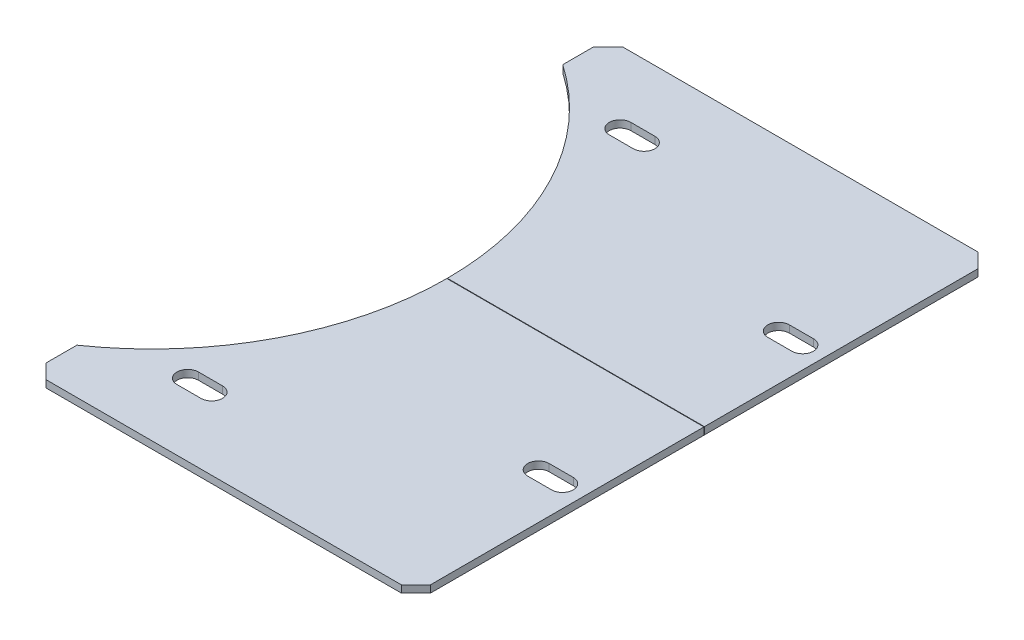
SolidWorks part; units mm, degrees
ref_plane "Front Plane" through (0, 0, 0) normal (0, 0, 1) x (1, 0, 0)
ref_plane "Top Plane" through (0, 0, 0) normal (0, 1, 0) x (1, 0, 0)
ref_plane "Right Plane" through (0, 0, 0) normal (1, 0, 0) x (0, 0, -1)
sketch "Sketch1" plane through (0, 0, 0) normal (0, 1, 0) x (1, 0, 0)
  line L1 (-276, 60) -> (276, 60)
  line L2 (-276, 60) -> (-276, -60)
  line L3 (-276, -60) -> (276, -60)
  line L4 (276, 60) -> (276, -60)
  line L5 (-276, 60) -> (276, -60) construction
  line L6 (-276, -60) -> (276, 60) construction
  point P0 (0, 0)
  dimension "D1" = 120
  dimension "D2" = 552
extrude "Boss-Extrude1" add sketch "Sketch1" along normal blind 1.5
chamfer "Chamfer1" distance 3 angle 45 2 edges at (276, 0.75, -60) (276, 0.75, 60)
chamfer "Chamfer2" distance 3 angle 45 2 edges at (-276, 0.75, -60) (-276, 0.75, 60)
sketch "Sketch12" plane through (0, 1.5, 0) normal (0, 1, 0) x (1, 0, 0)
  line L0 (-258.5, 45) -> (-253.5, 45) construction
  line L1 (-258.5, 47.25) -> (-253.5, 47.25)
  line L2 (-258.5, 42.75) -> (-253.5, 42.75)
  line L3 (-258.5, -45) -> (-253.5, -45) construction
  line L4 (-258.5, -42.75) -> (-253.5, -42.75)
  line L5 (-258.5, -47.25) -> (-253.5, -47.25)
  line L6 (0, 0) -> (-462.1641, 0) construction
  line L7 (-276, 57) -> (-276, -57) construction
  line L8 (273, 60) -> (-273, 60) construction
  arc A0 (-258.5, 47.25) -> (-258.5, 42.75) centre (-258.5, 45) ccw
  arc A1 (-253.5, 42.75) -> (-253.5, 47.25) centre (-253.5, 45) ccw
  arc A2 (-258.5, -42.75) -> (-258.5, -47.25) centre (-258.5, -45) ccw
  arc A3 (-253.5, -47.25) -> (-253.5, -42.75) centre (-253.5, -45) ccw
  point P2 (-256, 45)
  point P7 (-256, -45)
  dimension "D1" = 4.5
  dimension "D2" = 5
  dimension "D3" = 20
  dimension "D4" = 15
extrude "Cut-Extrude6" cut sketch "Sketch12" against normal through all
sketch "Sketch13" plane through (0, 1.5, 0) normal (0, 1, 0) x (1, 0, 0)
  line L0 (276, -57) -> (276, 57) construction
  line L1 (-276, 0.05) -> (276, 0.05)
  line L2 (-276, 0.05) -> (-276, -0.05)
  line L3 (-276, -0.05) -> (276, -0.05)
  line L4 (276, 0.05) -> (276, -0.05)
  line L5 (-276, 0.05) -> (276, -0.05) construction
  line L6 (-276, -0.05) -> (276, 0.05) construction
  line L7 (-276, 57) -> (-276, -57) construction
  point P0 (0, 0)
  dimension "D1" = 0.1
extrude "Cut-Extrude7" cut sketch "Sketch13" against normal through all
sketch "Sketch15" plane through (0, 1.5, 0) normal (0, 1, 0) x (1, 0, 0)
  line L0 (-276, -0.05) -> (276, -0.05) construction
  line L1 (52, 35.95) -> (-14, 35.95)
  line L2 (55, 32.95) -> (55, -33.05)
  line L3 (52, -36.05) -> (-14, -36.05)
  line L4 (-17, 32.95) -> (-17, -33.05)
  line L5 (55, 35.95) -> (-17, -36.05) construction
  line L6 (55, -36.05) -> (-17, 35.95) construction
  line L7 (-276, 57) -> (-276, 0.05) construction
  arc A0 (-17, -33.05) -> (-14, -36.05) centre (-14, -33.05) ccw
  arc A1 (55, -33.05) -> (52, -36.05) centre (52, -33.05) cw
  arc A2 (55, 32.95) -> (52, 35.95) centre (52, 32.95) ccw
  arc A3 (-14, 35.95) -> (-17, 32.95) centre (-14, 32.95) ccw
  point P0 (19, -0.05)
  dimension "D3" = 3
  dimension "D1" = 72
  dimension "D2" = 72
  dimension "D4" = 295
extrude "Cut-Extrude9" cut sketch "Sketch15" against normal through all
sketch "Sketch16" plane through (0, 1.5, 0) normal (0, 1, 0) x (1, 0, 0)
  line L0 (276, 0.05) -> (276, 57) construction
  line L1 (0, 0) -> (352.5911, 0) construction
  line L2 (0, 0) -> (0, 143.0362) construction
  circle A0 centre (311, 0) radius 61.5
  circle A1 centre (-311, 0) radius 61.5
  dimension "D1" = 123
  dimension "D2" = 35
extrude "Cut-Extrude10" cut sketch "Sketch16" against normal blind 10
sketch "Sketch17" plane through (0, 0, 0) normal (0, -1, 0) x (1, 0, 0)
  line L0 (-200.5, -25) -> (-205.5, -25) construction
  line L1 (-200.5, -27.25) -> (-205.5, -27.25)
  line L2 (-200.5, -22.75) -> (-205.5, -22.75)
  line L3 (-200.5, 25) -> (-205.5, 25) construction
  line L4 (-200.5, 22.75) -> (-205.5, 22.75)
  line L5 (-200.5, 27.25) -> (-205.5, 27.25)
  line L6 (-203, -60) -> (-203, 60) construction
  line L8 (273, -60) -> (-273, -60) construction
  line L9 (-273, 60) -> (273, 60) construction
  line L10 (-311, 0) -> (-268.0046, 0) construction
  line L11 (-276, -57) -> (-276, -50.5693) construction
  arc A0 (-200.5, -27.25) -> (-200.5, -22.75) centre (-200.5, -25) ccw
  arc A1 (-205.5, -22.75) -> (-205.5, -27.25) centre (-205.5, -25) ccw
  arc A2 (-200.5, 22.75) -> (-200.5, 27.25) centre (-200.5, 25) ccw
  arc A3 (-205.5, 27.25) -> (-205.5, 22.75) centre (-205.5, 25) ccw
  point P2 (-203, -25)
  point P7 (-203, 25)
  dimension "D1" = 5
  dimension "D2" = 4.5
  dimension "D3" = 50
  dimension "D4" = 73
sketch "Sketch18" plane through (0, 0, 0) normal (0, -1, 0) x (1, 0, 0)
  line L0 (-276, -57) -> (-276, -50.5693) construction
  line L1 (802.7899, 126.4319) -> (-196, 126.4319)
  line L2 (802.7899, 126.4319) -> (802.7899, -126.4319)
  line L3 (802.7899, -126.4319) -> (-196, -126.4319)
  line L4 (-196, 126.4319) -> (-196, -126.4319)
  line L5 (802.7899, 126.4319) -> (-196, -126.4319) construction
  line L6 (802.7899, -126.4319) -> (-196, 126.4319) construction
  point P0 (303.3949, 0)
  dimension "D1" = 80
extrude "Cut-Extrude11" cut sketch "Sketch18" against normal blind 10
extrude "Cut-Extrude12" cut sketch "Sketch17" against normal blind 10
chamfer "Chamfer3" distance 3 angle 45 1 edges at (-196, 0.75, 60)
chamfer "Chamfer4" distance 3 angle 45 1 edges at (-196, 0.75, -60)
